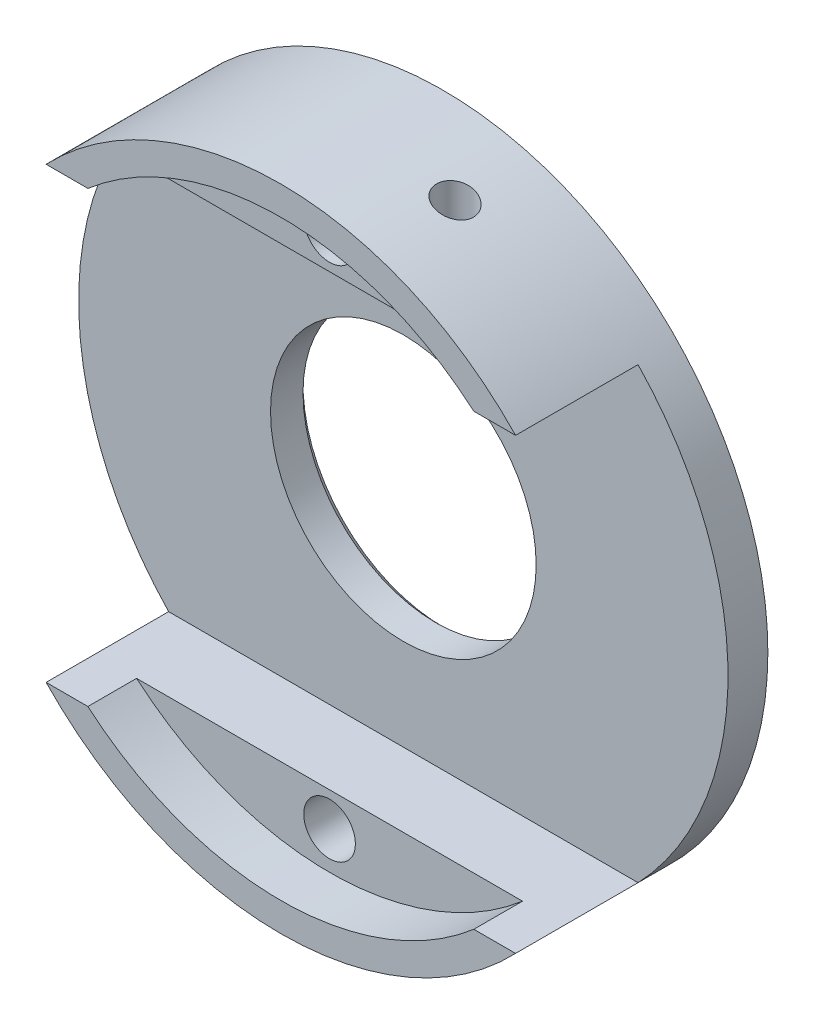
from build123d import *

# Parameters (mm, degrees)
SKETCH1_R           = 22
BOSS_EXTRUDE1_DEPTH = 11
SKETCH2_R           = 20.05
CUT_EXTRUDE1_DEPTH  = 8.3
SKETCH3_W           = 67.682797152
SKETCH3_H           = 30.4
CUT_EXTRUDE2_DEPTH  = 8.3
SKETCH4_R           = 1.75
CUT_EXTRUDE3_DEPTH  = 5
CIRPATTERN1_COUNT   = 2
CUT_EXTRUDE4_REACH  = 35
SKETCH5_R           = 9
CHAMFER1_SIZE       = 1.5
CHAMFER2_SIZE       = 0.5
SKETCH6_OUTSIDE_W   = 58.638
SKETCH6_OUTSIDE_H   = 58.638
SKETCH6_OUTSIDE_W_2 = 90.952157774
SKETCH6_OUTSIDE_H_2 = 47
CUT_EXTRUDE5_DEPTH  = 8.3
BOSS_EXTRUDE2_START = 5
SKETCH7_R           = 1.75
BOSS_EXTRUDE2_DEPTH = 5
SKETCH8_R           = 1.25
CUT_EXTRUDE6_DEPTH  = 11


with BuildPart() as part:
    # Sketch1 → Boss-Extrude1 (new body)
    with BuildSketch(Plane.XY):
        Circle(SKETCH1_R)
    extrude(amount=BOSS_EXTRUDE1_DEPTH)

    # Sketch2 → Cut-Extrude1 (cut)
    with BuildSketch(Plane.XY.offset(11)):
        Circle(SKETCH2_R)
    extrude(amount=-CUT_EXTRUDE1_DEPTH, mode=Mode.SUBTRACT)

    # Sketch3 → Cut-Extrude2 (cut)
    with BuildSketch(Plane.XY.offset(2.7)):
        Rectangle(SKETCH3_W, SKETCH3_H)
    extrude(amount=CUT_EXTRUDE2_DEPTH, mode=Mode.SUBTRACT)

    # Sketch4 → Cut-Extrude3 (cut)
    with BuildSketch(Plane(origin=(0, 0, 0), x_dir=(-1, 0, 0), z_dir=(0, 0, -1))):
        with Locations((0, 17.5)):
            Circle(SKETCH4_R)
    cut_extrude3 = extrude(amount=-CUT_EXTRUDE3_DEPTH, mode=Mode.SUBTRACT)

    # CirPattern1: Cut-Extrude3 ×2 about axis
    cirpattern1_axis = Axis((0, 0, 0), (0, 0, 1))
    for i in range(1, CIRPATTERN1_COUNT):
        add(cut_extrude3.rotate(cirpattern1_axis, i * 360 / CIRPATTERN1_COUNT), mode=Mode.SUBTRACT)

    # Sketch5 → Cut-Extrude4 (cut, up to next)
    with BuildSketch(Plane(origin=(0, 0, 0), x_dir=(-1, 0, 0), z_dir=(0, 0, -1)), mode=Mode.PRIVATE) as cut_extrude4_sk1:
        Circle(SKETCH5_R)
    cut_extrude4_tool1 = extrude(cut_extrude4_sk1.sketch, amount=-CUT_EXTRUDE4_REACH, mode=Mode.PRIVATE) & part.part
    add(cut_extrude4_tool1.solids().sort_by_distance((0, 0, 0))[0], mode=Mode.SUBTRACT)

    # Chamfer1
    chamfer1_edges = [part.edges().sort_by_distance(p)[0] for p in [
        (1.75, 17.5, 0),
        (-1.75, -17.5, 0),
    ]]
    chamfer(chamfer1_edges, length=CHAMFER1_SIZE)

    # Chamfer2
    chamfer2_edges = [part.edges().sort_by_distance(p)[0] for p in [
        (9, 0, 0),
    ]]
    chamfer(chamfer2_edges, length=CHAMFER2_SIZE)

    # Sketch6 outside → Cut-Extrude5 (cut)
    with BuildSketch(Plane.XY.offset(11)):
        Rectangle(SKETCH6_OUTSIDE_W, SKETCH6_OUTSIDE_H)
        Rectangle(SKETCH6_OUTSIDE_W_2, SKETCH6_OUTSIDE_H_2, mode=Mode.SUBTRACT)
    extrude(amount=-CUT_EXTRUDE5_DEPTH, mode=Mode.SUBTRACT)

    # Sketch7 → Boss-Extrude2 (add)
    # profile 1 of 2: a face of its own
    with BuildSketch(Plane.XY.offset(2.7).offset(BOSS_EXTRUDE2_START)):
        with BuildLine():
            Line((-13.075262904, 15.2), (13.075262904, 15.2))
            ThreePointArc((13.075262904, 15.2), (0, 20.05), (-13.075262904, 15.2))
        make_face()
        with Locations((0, 17.5)):
            Circle(SKETCH7_R, mode=Mode.SUBTRACT)
    # profile 2 of 2: a face of its own
    with BuildSketch(Plane.XY.offset(2.7).offset(BOSS_EXTRUDE2_START)):
        with BuildLine():
            Line((-13.075262904, -15.2), (13.075262904, -15.2))
            ThreePointArc((13.075262904, -15.2), (0, -20.05), (-13.075262904, -15.2))
        make_face()
        with Locations((0, -17.5)):
            Circle(SKETCH7_R, mode=Mode.SUBTRACT)
    extrude(amount=-BOSS_EXTRUDE2_DEPTH)

    # Sketch8 → Cut-Extrude6 (cut)
    with BuildSketch(Plane.XZ.offset(-15.2)):
        with Locations(Location((6, 5.2, 0), (0, 0, 270))):
            Circle(SKETCH8_R)
    extrude(amount=-CUT_EXTRUDE6_DEPTH, mode=Mode.SUBTRACT)


solid = part.part
